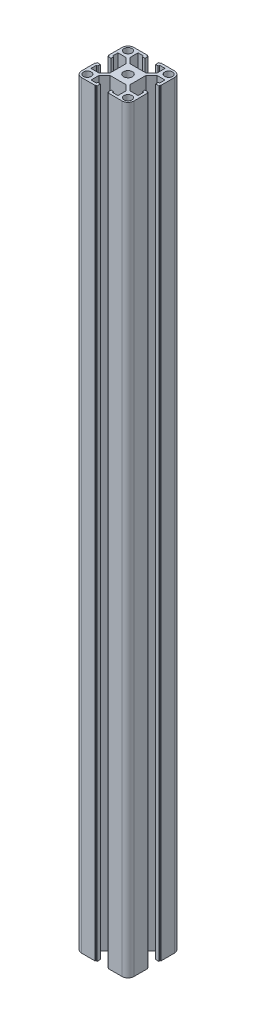
SolidWorks part; units mm, degrees
ref_plane "主视基准图" through (0, 0, 0) normal (0, 0, 1) x (1, 0, 0)
ref_plane "上视基准图" through (0, 0, 0) normal (0, 1, 0) x (1, 0, 0)
ref_plane "右视基准图" through (0, 0, 0) normal (1, 0, 0) x (0, 0, -1)
sketch "草图1" plane through (0, 0, 0) normal (0, 0, 1) x (1, 0, 0)
  line L0 (0, 0) -> (0, 580)
  dimension "D1" = 580
other "结构构件1"
ref_plane "基准面1" through (0, 0, 0) normal (0, 1, 0) x (-1, 0, 0)
sketch "Sketch16" plane through (0, 0, 0) normal (0, 1, 0) x (-1, 0, 0)
  line L0 (-5.1, 20) -> (-5.1, 19.5)
  line L1 (-5.1, 19.5) -> (-4.1, 19.5)
  line L2 (-4.1, 19.5) -> (-4.1, 17)
  line L3 (-6.1, 18) -> (-10.3, 18)
  line L4 (-15.5, -20) -> (-5.1, -20)
  line L5 (-20, -15.5) -> (-20, -5.1)
  line L6 (15.5, 20) -> (5.1, 20)
  line L7 (20, 15.5) -> (20, 5.1)
  line L8 (0, 14.8756) -> (0, 0) construction
  line L9 (0, 0) -> (14.1675, 0) construction
  line L10 (-10.3, 18) -> (-10.3, 12)
  line L11 (-10.3, 12) -> (-6, 7.7)
  line L12 (-6, 7.7) -> (6, 7.7)
  line L13 (10.3, 12) -> (6, 7.7)
  line L14 (10.3, 18) -> (10.3, 12)
  line L15 (6.1, 18) -> (10.3, 18)
  line L16 (4.1, 19.5) -> (4.1, 17)
  line L17 (5.1, 19.5) -> (4.1, 19.5)
  line L18 (5.1, 20) -> (5.1, 19.5)
  line L19 (-5.1, 20) -> (-15.5, 20)
  line L20 (20, 5.1) -> (19.5, 5.1)
  line L21 (0, 0) -> (-15.5563, 15.5563) construction
  line L22 (0, 0) -> (-15.5563, -15.5563) construction
  line L25 (19.5, 5.1) -> (19.5, 4.1)
  line L26 (19.5, 4.1) -> (17, 4.1)
  line L27 (17, 6.1) -> (17, 4.1)
  line L28 (18, 6.1) -> (17, 6.1)
  line L29 (18, 6.1) -> (18, 10.3)
  line L30 (18, 10.3) -> (12, 10.3)
  line L31 (12, 10.3) -> (7.7, 6)
  line L32 (7.7, 6) -> (7.7, -6)
  line L33 (12, -10.3) -> (7.7, -6)
  line L34 (18, -10.3) -> (12, -10.3)
  line L35 (18, -6.1) -> (18, -10.3)
  line L36 (18, -6.1) -> (17, -6.1)
  line L37 (17, -4.1) -> (17, -6.1)
  line L38 (19.5, -4.1) -> (17, -4.1)
  line L39 (19.5, -5.1) -> (19.5, -4.1)
  line L40 (20, -5.1) -> (19.5, -5.1)
  line L41 (5.1, -20) -> (5.1, -19.5)
  line L42 (5.1, -19.5) -> (4.1, -19.5)
  line L43 (4.1, -19.5) -> (4.1, -17)
  line L44 (6.1, -17) -> (4.1, -17)
  line L45 (6.1, -18) -> (6.1, -17)
  line L46 (6.1, -18) -> (10.3, -18)
  line L47 (10.3, -18) -> (10.3, -12)
  line L48 (10.3, -12) -> (6, -7.7)
  line L49 (6, -7.7) -> (-6, -7.7)
  line L50 (-10.3, -12) -> (-6, -7.7)
  line L51 (-10.3, -18) -> (-10.3, -12)
  line L52 (-6.1, -18) -> (-10.3, -18)
  line L53 (-6.1, -18) -> (-6.1, -17)
  line L54 (-4.1, -17) -> (-6.1, -17)
  line L55 (-4.1, -19.5) -> (-4.1, -17)
  line L56 (-5.1, -19.5) -> (-4.1, -19.5)
  line L57 (-5.1, -20) -> (-5.1, -19.5)
  line L58 (-20, -5.1) -> (-19.5, -5.1)
  line L59 (5.1, -20) -> (15.5, -20)
  line L60 (-20, 5.1) -> (-20, 15.5)
  line L61 (-19.5, -5.1) -> (-19.5, -4.1)
  line L62 (-6.1, 18) -> (-6.1, 17)
  line L63 (-6.1, 17) -> (-4.1, 17)
  line L64 (6.1, 18) -> (6.1, 17)
  line L65 (4.1, 17) -> (6.1, 17)
  line L66 (-19.5, -4.1) -> (-17, -4.1)
  line L71 (-17, -6.1) -> (-17, -4.1)
  line L72 (-18, -6.1) -> (-17, -6.1)
  line L73 (-18, -6.1) -> (-18, -10.3)
  line L74 (-18, -10.3) -> (-12, -10.3)
  line L75 (-12, -10.3) -> (-7.7, -6)
  line L76 (-7.7, -6) -> (-7.7, 6)
  line L77 (-12, 10.3) -> (-7.7, 6)
  line L78 (-18, 10.3) -> (-12, 10.3)
  line L79 (-18, 6.1) -> (-18, 10.3)
  line L80 (-18, 6.1) -> (-17, 6.1)
  line L81 (-17, 4.1) -> (-17, 6.1)
  line L82 (-19.5, 4.1) -> (-17, 4.1)
  line L83 (-19.5, 5.1) -> (-19.5, 4.1)
  line L84 (-20, 5.1) -> (-19.5, 5.1)
  line L85 (20, -5.1) -> (20, -15.5)
  circle A0 centre (0, 0) radius 3.4
  arc A1 (-20, 15.5) -> (-15.5, 20) centre (-15.5, 15.5) cw
  arc A2 (20, 15.5) -> (15.5, 20) centre (15.5, 15.5) ccw
  arc A3 (-15.5, -20) -> (-20, -15.5) centre (-15.5, -15.5) cw
  arc A4 (15.5, -20) -> (20, -15.5) centre (15.5, -15.5) ccw
  circle A5 centre (-15.5563, 15.5563) radius 3
  circle A6 centre (15.5563, 15.5563) radius 3
  circle A7 centre (15.5563, -15.5563) radius 3
  circle A8 centre (-15.5563, -15.5563) radius 3
  point P2 (0, 10)
  point P3 (0, 0)
  point P4 (0, 0)
  point P5 (-20, -20)
  point P6 (20, -20)
  point P7 (20, 20)
  point P8 (-20, 20)
  point P36 (-20, 20)
  point P39 (20, 20)
  dimension "D1" = 20.6
  dimension "D2" = 40
  dimension "D3" = 8.2
  dimension "D4" = 10.2
  dimension "D5" = 12.3
  dimension "D6" = 6.8
  dimension "D7" = 4.5
  dimension "D8" = 45
  dimension "D12" = 6
  dimension "D13" = 22
  dimension "D9" = 0.5
  dimension "D10" = 2
  dimension "D11" = 12
  dimension "D16" = 3
  dimension "D17" = 2
